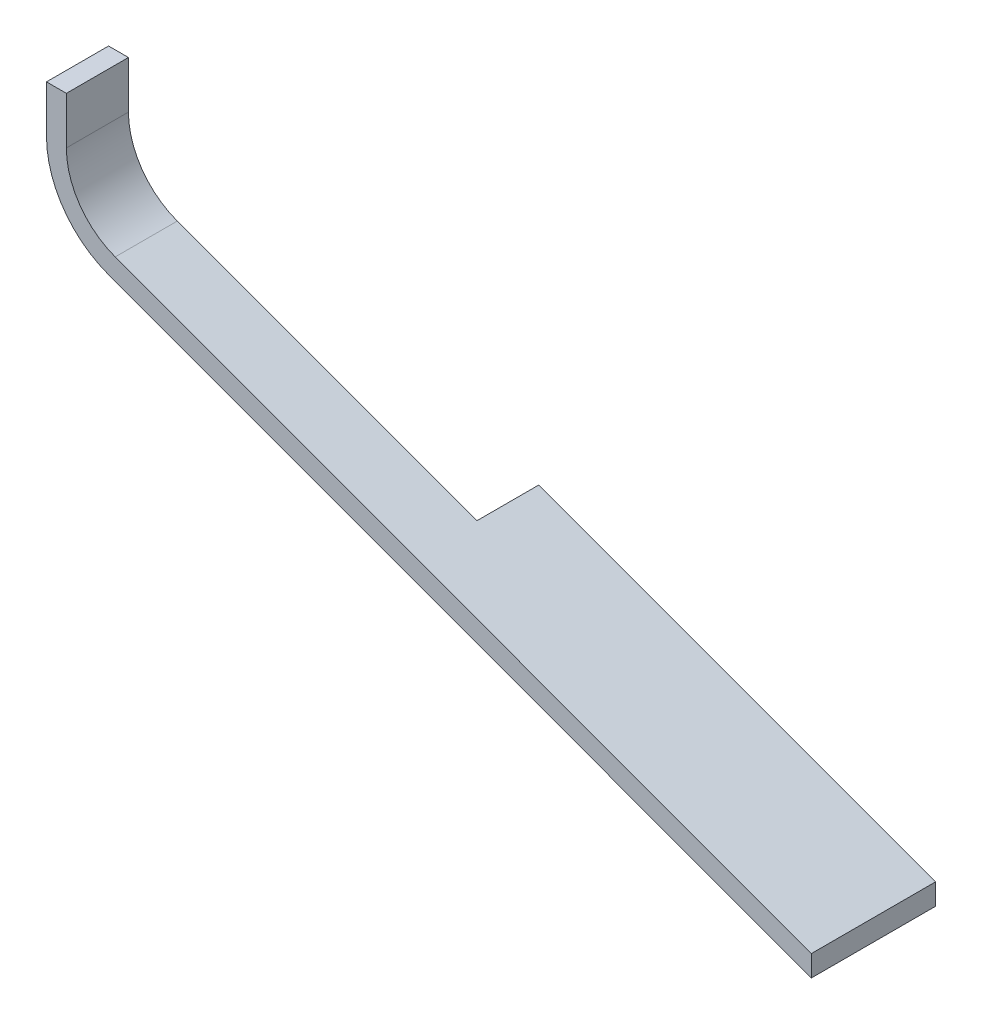
from build123d import *

# Parameters (mm, degrees)
EXTRUDE_1_DEPTH     = 50
SKETCH_2_W          = 128.455604429
SKETCH_2_H          = 25
SKETCH_2_W_2        = 42.23428711
CUT_EXTRUDE_2_DEPTH = 50


with BuildPart() as part:
    # 草图1 → 凸台-拉伸1 (new body)
    with BuildSketch(Plane.XY):
        with BuildLine():
            Line((-158.499845276, 75.499845276), (-158.499845276, 56.452935893))
            ThreePointArc((-158.499845276, 56.452935893), (-151.653526546, 34.694072336), (-133.581521944, 20.77563589))
            Line((-133.581521944, 20.77563589), (146.746117531, -82.011165251))
            Line((146.746117531, -82.011165251), (149.500154724, -83.020978889))
            Line((149.500154724, -83.020978889), (149.500154724, -74.500154724))
            Line((149.500154724, -74.500154724), (-130.827484751, 28.286646417))
            ThreePointArc((-130.827484751, 28.286646417), (-145.094856805, 39.274885717), (-150.499845276, 56.452935893))
            Line((-150.499845276, 56.452935893), (-150.499845276, 75.499845276))
            Line((-150.499845276, 75.499845276), (-158.499845276, 75.499845276))
        make_face()
    extrude(amount=EXTRUDE_1_DEPTH)

    # 草图2 → 切除-拉伸2 (cut)
    with BuildSketch(Plane(origin=(-9.115968963, -24.861733537, 0), x_dir=(0.9388763158866098, -0.3442546491584201, 0), z_dir=(-0.3442546491584201, -0.9388763158866098, 0))):
        with Locations((-68.340834223, 12.5)):
            Rectangle(SKETCH_2_W, SKETCH_2_H)
        with Locations((-153.685779993, 12.5)):
            Rectangle(SKETCH_2_W_2, SKETCH_2_H)
    extrude(amount=-CUT_EXTRUDE_2_DEPTH, mode=Mode.SUBTRACT)


solid = part.part
